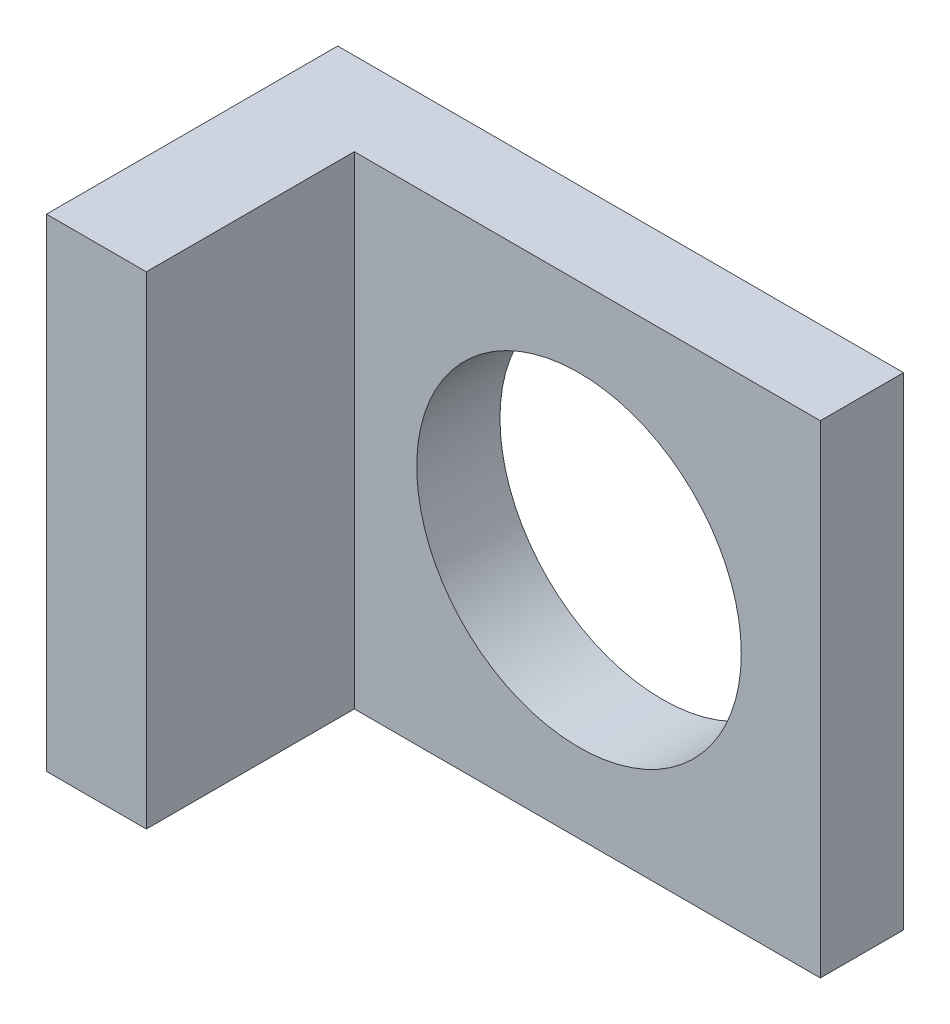
SolidWorks part; units mm, degrees
ref_plane "前视基准面" through (0, 0, 0) normal (0, 0, 1) x (1, 0, 0)
ref_plane "上视基准面" through (0, 0, 0) normal (0, 1, 0) x (1, 0, 0)
ref_plane "右视基准面" through (0, 0, 0) normal (1, 0, 0) x (0, 0, -1)
sketch "草图1" plane through (0, 0, 0) normal (0, 0, 1) x (1, 0, 0)
  line L0 (0, 0) -> (0, 58)
  line L1 (0, 58) -> (68, 58)
  line L2 (68, 58) -> (68, 0)
  line L3 (68, 0) -> (0, 0)
  point P6 (0, -1.223)
  dimension "D3" = 58
  dimension "D4" = 68
extrude "凸台-拉伸1" add sketch "草图1" along normal blind 10
sketch "草图2" plane through (0, 0, 10) normal (0, 0, 1) x (1, 0, 0)
  line L0 (68, 0) -> (68, 58) construction
  line L1 (0, 0) -> (68, 0) construction
  circle A0 centre (39, 29) radius 19.5
  dimension "D1" = 39
  dimension "D2" = 29
  dimension "D3" = 29
extrude "切除-拉伸1" cut sketch "草图2" against normal up to next
sketch "草图3" plane through (0, 0, 0) normal (0, 0, -1) x (-1, 0, 0)
  line L1 (0, 0) -> (-12, 0)
  line L2 (0, 0) -> (0, 30)
  line L3 (0, 30) -> (-12, 30)
  line L4 (-12, 0) -> (-12, 30)
  dimension "D1" = 30
  dimension "D2" = 12
extrude "凸台-拉伸2" [suppressed] add sketch "草图3" along normal blind 37
sketch "草图4" plane through (0, 0, 10) normal (0, 0, 1) x (1, 0, 0)
  line L0 (0, 0) -> (68, 0) construction
  line L1 (0, 58) -> (12, 58)
  line L2 (0, 58) -> (0, 0)
  line L3 (0, 0) -> (12, 0)
  line L4 (12, 58) -> (12, 0)
  dimension "D1" = 12
extrude "凸台-拉伸3" add sketch "草图4" along normal blind 25
